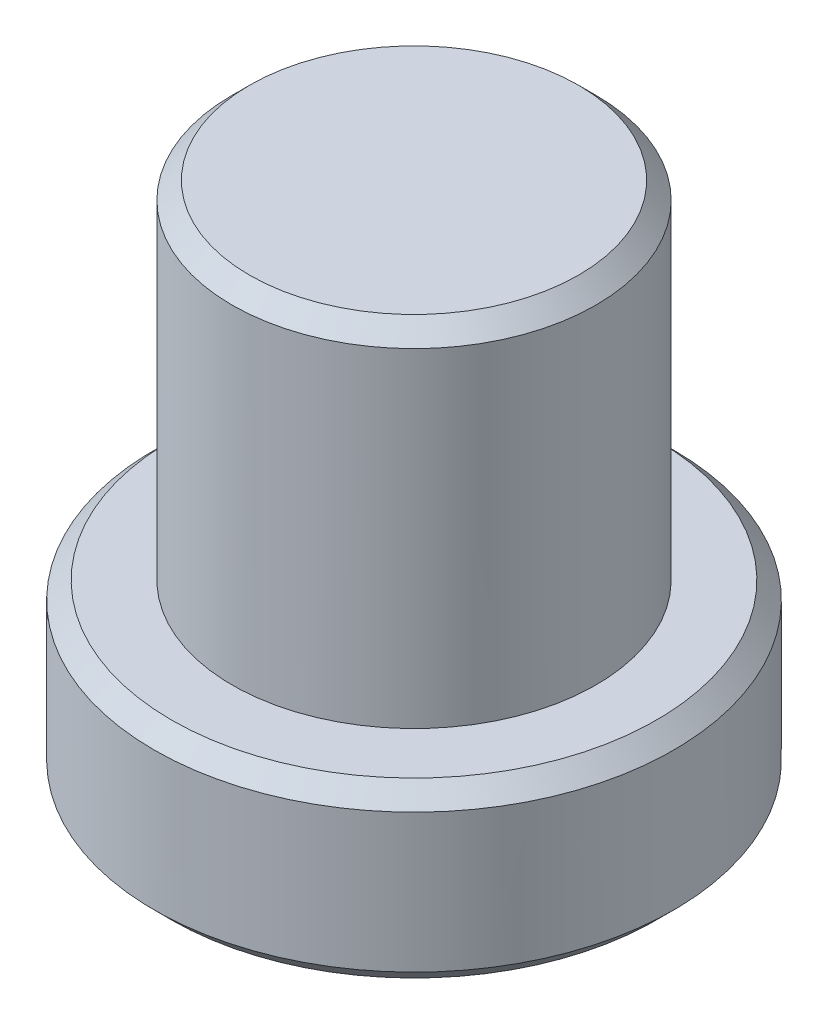
SolidWorks part; units mm, degrees
material "20#"
ref_plane "Front Plane" through (0, 0, 0) normal (0, 0, 1) x (1, 0, 0)
ref_plane "Top Plane" through (0, 0, 0) normal (0, 1, 0) x (1, 0, 0)
ref_plane "Right Plane" through (0, 0, 0) normal (1, 0, 0) x (0, 0, -1)
sketch "Sketch1" plane through (0, 0, 0) normal (1, 0, 0) x (0, 0, -1)
  line L0 (0, 0) -> (0, 15) construction
  line L1 (0, 15) -> (5.25, 15)
  line L2 (5.25, 15) -> (5.25, 5)
  line L3 (5.25, 5) -> (7.5, 5)
  line L4 (7.5, 5) -> (7.5, 0)
  line L5 (7.5, 0) -> (0, 0)
  line L6 (0, 0) -> (0, 15)
  dimension "D1" = 5
  dimension "D2" = 10
  dimension "D3" = 10.5
  dimension "D4" = 15
revolve "Revolve1" add sketch "Sketch1" angle 360 about L0
chamfer "Chamfer1" distance 0.5 angle 45 3 edges at (0, 0, -7.5) (0, 5, -7.5) (0, 15, -5.25)
